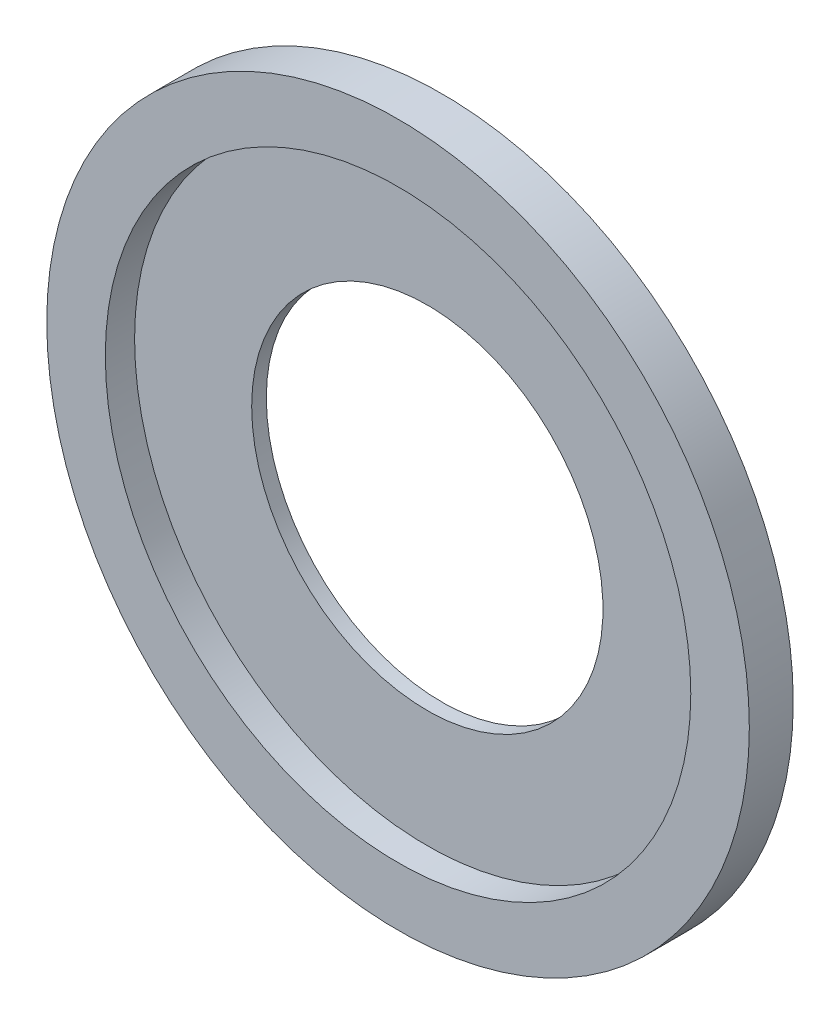
from build123d import *

# Parameters (mm, degrees)
SKETCH_1_R          = 60
SKETCH_1_R_2        = 50
EXTRUDE_1_DEPTH     = 7.5
SKETCH_2_R          = 50
SKETCH_2_R_2        = 20
EXTRUDE_2_DEPTH     = 2.5
SKETCH_4_R          = 30
CUT_EXTRUDE_1_DEPTH = 10


with BuildPart() as part:
    # 草图1 → 拉伸1 (new body)
    with BuildSketch(Plane.XY):
        Circle(SKETCH_1_R)
        Circle(SKETCH_1_R_2, mode=Mode.SUBTRACT)
    extrude(amount=EXTRUDE_1_DEPTH)

    # 草图2 → 拉伸2 (add)
    with BuildSketch(Plane(origin=(0, 0, 0), x_dir=(-1, 0, 0), z_dir=(0, 0, -1))):
        Circle(SKETCH_2_R)
        Circle(SKETCH_2_R_2, mode=Mode.SUBTRACT)
    extrude(amount=-EXTRUDE_2_DEPTH)

    # 草图4 → 切除-拉伸1 (cut)
    with BuildSketch(Plane(origin=(0, 0, 0), x_dir=(-1, 0, 0), z_dir=(0, 0, -1))):
        Circle(SKETCH_4_R)
    extrude(amount=-CUT_EXTRUDE_1_DEPTH, mode=Mode.SUBTRACT)


solid = part.part
